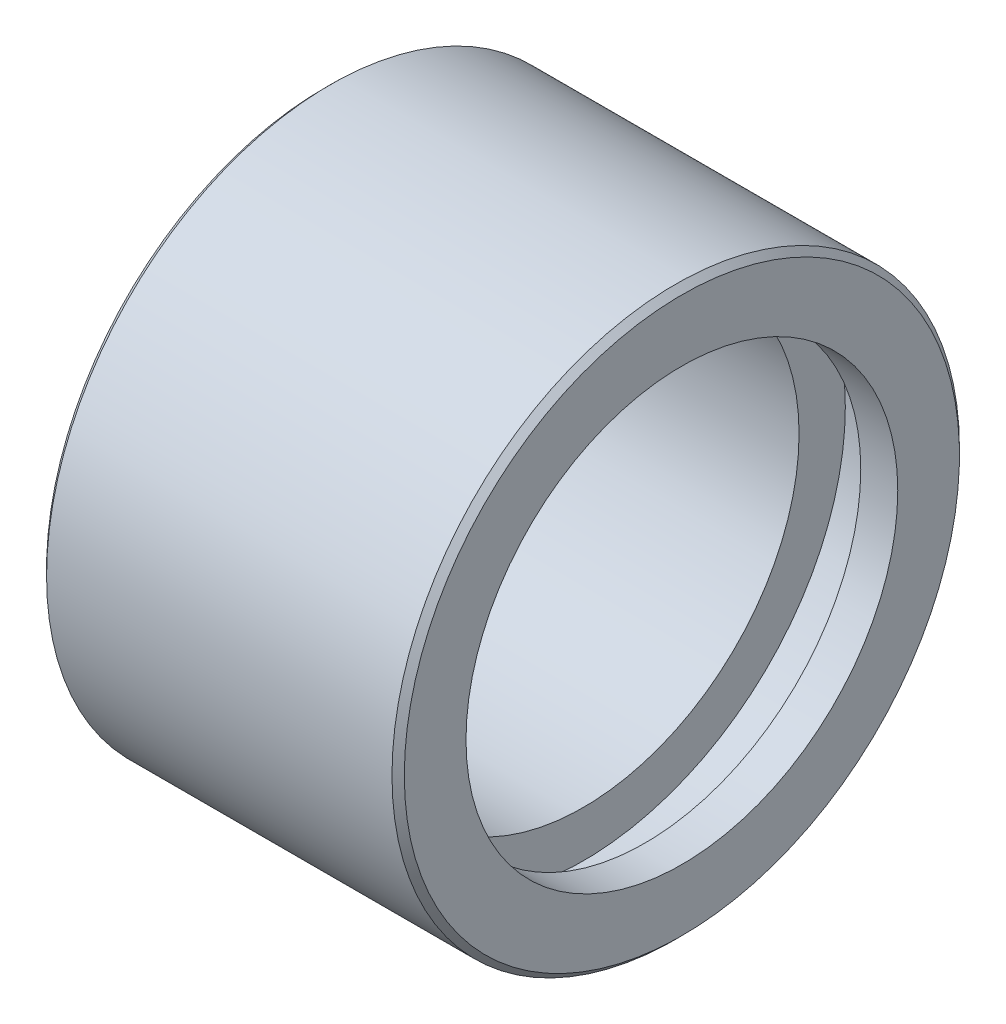
SolidWorks part; units mm, degrees
ref_plane "前视基准面" through (0, 0, 0) normal (0, 0, 1) x (1, 0, 0)
ref_plane "上视基准面" through (0, 0, 0) normal (0, 1, 0) x (1, 0, 0)
ref_plane "右视基准面" through (0, 0, 0) normal (1, 0, 0) x (0, 0, -1)
sketch "草图1" plane through (0, 0, 0) normal (0, 0, 1) x (1, 0, 0)
  line L0 (0, 0) -> (55.4911, 0) construction
  line L1 (0, 17.5) -> (21, 17.5)
  line L2 (21, 17.5) -> (21, 21.25)
  line L3 (21, 21.25) -> (26, 21.25)
  line L4 (26, 21.25) -> (26, 17.5)
  line L5 (26, 17.5) -> (29, 17.5)
  line L6 (29, 17.5) -> (29, 23)
  line L7 (0, 17.5) -> (0, 23)
  line L8 (0, 23) -> (29, 23)
  dimension "D1" = 17.5
  dimension "D2" = 90
  dimension "D3" = 3.75
  dimension "D4" = 17.5
  dimension "D5" = 21
  dimension "D6" = 5
  dimension "D7" = 3
  dimension "D8" = 5.5
revolve "旋转1" add sketch "草图1" angle 360 about L0
chamfer "倒角1" distance 0.5 angle 45 2 edges at (29, 0, 23) (0, 0, 23)
